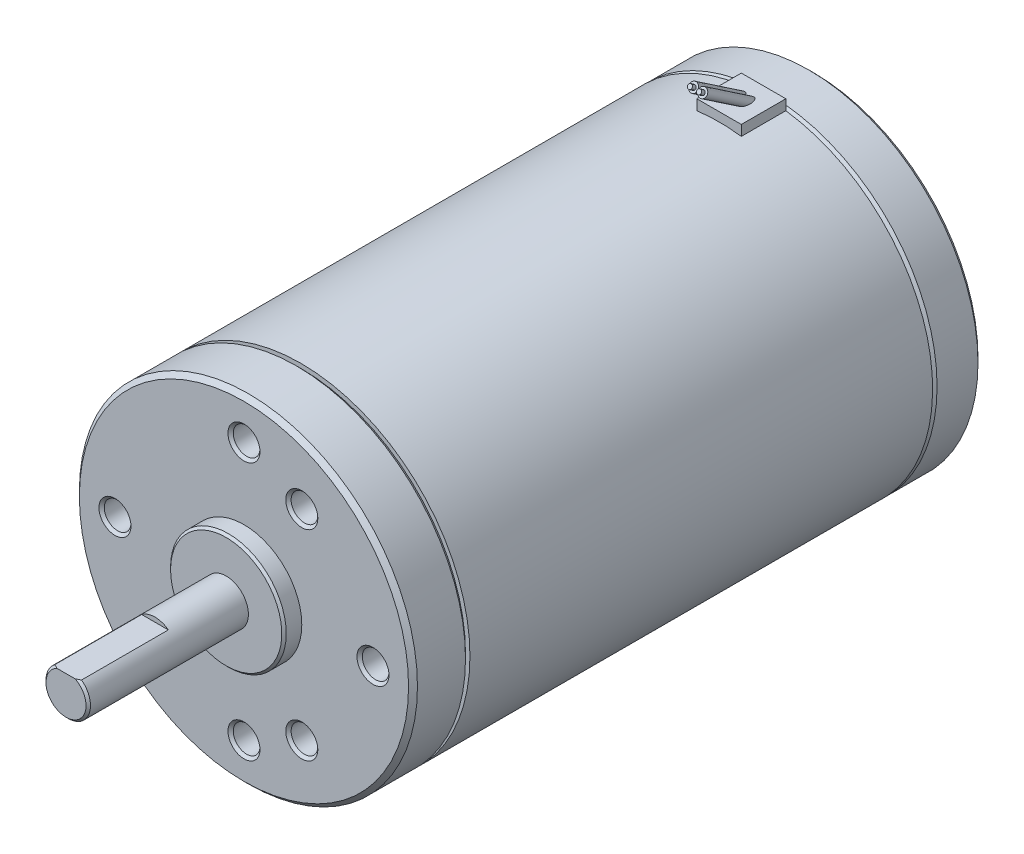
from build123d import *

# Parameters (mm, degrees)
SKETCH_13_W         = 5.6
SKETCH_13_H         = 19
SKETCH_2_W          = 52
SKETCH_2_H          = 19
SKETCH_15_W         = 18
SKETCH_15_H         = 2.5
SKETCH_17_W         = 10
SKETCH_17_H         = 0.5
CUT_EXTRUDE_1_DEPTH = 5
SKETCH_9_W          = 5
SKETCH_9_H          = 5
EXTRUDE_1_DEPTH     = 20
CHAMFER_1_SIZE      = 0.5
CHAMFER_2_SIZE      = 0.5
CHAMFER_3_SIZE      = 0.25
SKETCH_18_R         = 1.5
CUT_EXTRUDE_2_DEPTH = 6.4
CHAMFER_4_SIZE      = 0.3


with BuildPart() as part:
    # 草图13 → 旋转9 (revolve)
    with BuildSketch(Plane(origin=(0, 0, 0), x_dir=(0, 0, -1), z_dir=(1, 0, 0)), mode=Mode.PRIVATE) as revolve_9_sk:
        Polygon((0, 19), (6.4, 19), (6.4, 0), (0, 0), (-2, 0), (-2, 6.5), (0, 6.5), align=None)
        with Locations((61.2, 9.5)):
            Rectangle(SKETCH_13_W, SKETCH_13_H)
    revolve(revolve_9_sk.sketch.rotate(Axis((0, 0, -58.4), (0, 0, -1)), 90), axis=Axis((0, 0, -58.4), (0, 0, -1)))

    # 草图15 → 旋转11 (revolve)
    with BuildSketch(Plane(origin=(0, 0, 0), x_dir=(0, 0, -1), z_dir=(1, 0, 0))):
        with Locations((-11, 1.25)):
            Rectangle(SKETCH_15_W, SKETCH_15_H)
    revolve(axis=Axis((0, 0, 2), (0, 0, 1)))

    # 草图17 → 切除-拉伸1 (cut, symmetric)
    with BuildSketch(Plane(origin=(0, 0, 0), x_dir=(0, 0, -1), z_dir=(1, 0, 0))):
        with Locations((-15, 2.25)):
            Rectangle(SKETCH_17_W, SKETCH_17_H)
    extrude(amount=CUT_EXTRUDE_1_DEPTH, both=True, mode=Mode.SUBTRACT)

    # 倒角1
    chamfer_1_edges = [part.edges().sort_by_distance(p)[0] for p in [
        (-19, 0, -58.4),
        (-19, 0, -64),
    ]]
    chamfer(chamfer_1_edges, length=CHAMFER_1_SIZE)

    # 倒角2
    chamfer_2_edges = [part.edges().sort_by_distance(p)[0] for p in [
        (-19, 0, -6.4),
        (-19, 0, 0),
    ]]
    chamfer(chamfer_2_edges, length=CHAMFER_2_SIZE)

    # 倒角3
    chamfer_3_edges = [part.edges().sort_by_distance(p)[0] for p in [
        (0, -2.5, 20),
        (-6.5, 0, 2),
    ]]
    chamfer(chamfer_3_edges, length=CHAMFER_3_SIZE)

    # 草图18 → 切除-拉伸2 (cut)
    with BuildSketch(Plane.XY):
        with Locations((0, 14.5)):
            Circle(SKETCH_18_R)
        with Locations((6.5, 11.258330249)):
            Circle(SKETCH_18_R)
        with Locations((6.5, -11.258330249)):
            Circle(SKETCH_18_R)
        with Locations((0, -14.5)):
            Circle(SKETCH_18_R)
        with Locations((14.5, 0)):
            Circle(SKETCH_18_R)
        with Locations((-14.5, 0)):
            Circle(SKETCH_18_R)
    extrude(amount=-CUT_EXTRUDE_2_DEPTH, mode=Mode.SUBTRACT)

    # 倒角4
    chamfer_4_edges = [part.edges().sort_by_distance(p)[0] for p in [
        (-1.5, 14.5, 0),
        (5, 11.258330249, 0),
        (5, -11.258330249, 0),
        (-1.5, -14.5, 0),
        (13, 0, 0),
        (-16, 0, 0),
    ]]
    chamfer(chamfer_4_edges, length=CHAMFER_4_SIZE)


with BuildPart() as body_2:
    # 草图2 → 旋转10 (revolve)
    with BuildSketch(Plane(origin=(0, 0, 0), x_dir=(0, 0, -1), z_dir=(1, 0, 0)), mode=Mode.PRIVATE) as revolve_10_sk:
        with Locations((32.4, 9.5)):
            Rectangle(SKETCH_2_W, SKETCH_2_H)
    revolve(revolve_10_sk.sketch.rotate(Axis((0, 0, -6.4), (0, 0, -1)), 180), axis=Axis((0, 0, -6.4), (0, 0, -1)))

    # 草图9 → 凸台-拉伸1 (add)
    with BuildSketch(Plane(origin=(0, 0, 0), x_dir=(1, 0, 0), z_dir=(0, 1, 0))):
        with Locations((0, 55.9)):
            Rectangle(SKETCH_9_W, SKETCH_9_H)
    extrude(amount=EXTRUDE_1_DEPTH)

    # 草图12 → 旋转12 (revolve)
    with BuildSketch(Plane(origin=(0.51, 0, 0), x_dir=(0, 0, -1), z_dir=(1, 0, 0))):
        Polygon((50.765931613, 22.869971904), (56.485742762, 19), (56.765931613, 19.414118591), (50.632001872, 23.564279347), (50.491907447, 23.357220051), (50.906026038, 23.0770312), align=None)
    revolve_12 = revolve(axis=Axis((0.51, 23.564279347, -50.632001872), (0, -0.5603777020527585, -0.8282371828420104)))

    # 镜向1: 旋转12 across plane
    add(revolve_12.mirror(Plane(origin=(0, 0, 0), x_dir=(0, 0, 1), z_dir=(1, 0, 0))))


solid = Compound([part.part, body_2.part])
